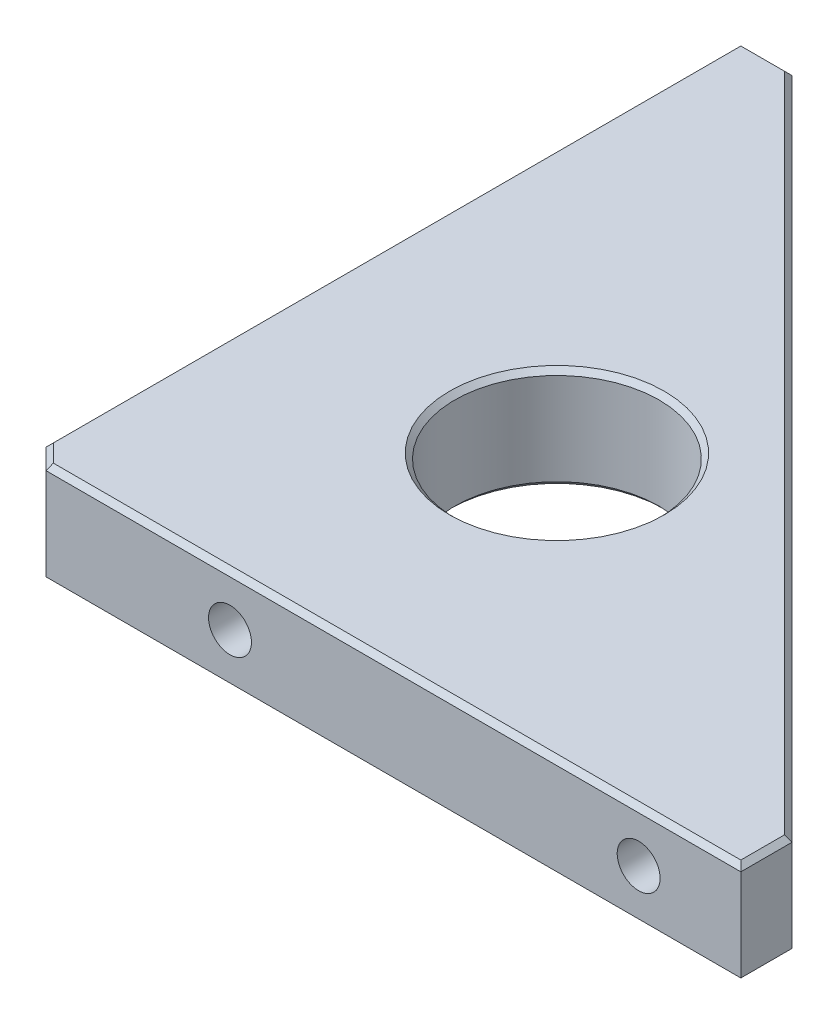
SolidWorks part; units mm, degrees
material "6061 合金"
ref_plane "前视" through (0, 0, 0) normal (0, 0, 1) x (1, 0, 0)
ref_plane "上视" through (0, 0, 0) normal (0, 1, 0) x (1, 0, 0)
ref_plane "右视" through (0, 0, 0) normal (1, 0, 0) x (0, 0, -1)
sketch "草图1" plane through (0, 0, 0) normal (0, 1, 0) x (1, 0, 0)
  line L0 (0, 0) -> (0, 70)
  line L1 (0, 70) -> (5, 70)
  line L2 (5, 70) -> (70, 5)
  line L3 (70, 5) -> (70, 0)
  line L4 (70, 0) -> (0, 0)
  dimension "D1" = 70
  dimension "D2" = 70
  dimension "D3" = 5
  dimension "D4" = 5
extrude "凸台-拉伸1" add sketch "草图1" along normal mid plane 10
chamfer "倒角1" distance 2 angle 45 1 edges at (0, 0, 0)
hole_wizard "M5 螺纹孔1" positions "草图2" profile "草图3" tap size "M5" standard "AS"
sketch "草图2" plane through (0, 0, 0) normal (0, 0, 1) x (1, 0, 0)
  line L0 (0, -5) -> (0, 5) construction
  line L1 (70, 5) -> (70, -5) construction
  point P0 (60, 0)
  point P2 (20, 0)
  dimension "D1" = 20
  dimension "D2" = 10
cosmetic thread "孔螺蚊线1" parameters "D1"=10, "D2"=5
cosmetic thread "孔螺蚊线2" parameters "D1"=10, "D2"=5
sketch "草图3" plane through (60, 0, 0) normal (1, 0, 0) x (0, -1, 0)
  line L0 (0, 0) -> (0, 13.6618)
  line L1 (0, 13.6618) -> (2.1, 12.4)
  line L2 (2.1, 12.4) -> (2.1, 0)
  line L5 (2.1, 0) -> (0, 0)
  line L10 (0, 13.6618) -> (-2.1, 12.4) construction
  line L11 (0, -6.35) -> (0, 107.95) construction
  dimension "螺纹孔钻头直径" = 4.2
  dimension "螺纹孔钻头深度" = 12.4
  dimension "导头角度" = 118
hole_wizard "M5 螺纹孔2" positions "草图4" profile "草图5" tap size "M5" standard "AS"
sketch "草图4" plane through (0, 0, 0) normal (-1, 0, 0) x (0, 0, 1)
  point P0 (-19.0545, 0)
  point P2 (-59.0545, 0)
  dimension "D1" = 19.0545
  dimension "D2" = 40
sketch "草图5" plane through (0, 0, -19.0545) normal (0, 1, 0) x (0, 0, 1)
  line L0 (0, 0) -> (0, 13.6618)
  line L1 (0, 13.6618) -> (2.1, 12.4)
  line L2 (2.1, 12.4) -> (2.1, 0)
  line L5 (2.1, 0) -> (0, 0)
  line L10 (0, 13.6618) -> (-2.1, 12.4) construction
  line L11 (0, -6.35) -> (0, 107.95) construction
  dimension "螺纹孔钻头直径" = 4.2
  dimension "螺纹孔钻头深度" = 12.4
  dimension "导头角度" = 118
cosmetic thread "孔螺蚊线6" parameters "D1"=10, "D2"=5
cosmetic thread "孔螺蚊线7" parameters "D1"=10, "D2"=5
sketch "草图6" plane through (0, -5, 0) normal (0, -1, 0) x (1, 0, 0)
  line L2 (0, -70) -> (0, -2) construction
  line L3 (2, 0) -> (70, 0) construction
  circle A0 centre (26, -26) radius 10
  dimension "D1" = 26
  dimension "D2" = 26
  dimension "D3" = 20
extrude "切除-拉伸1" cut sketch "草图6" against normal through all
chamfer "倒角2" distance 0.5 angle 45 14 edges at (70, -5, -2.5) (37.5, -5, -37.5) (2.5, -5, -70) (0, -5, -36) (1, -5, -1) (36, -5, 0) (2.5, 5, -70) (37.5, 5, -37.5) (70, 5, -2.5) (36, 5, 0) (1, 5, -1) (0, 5, -36) (26, -5, -36) (26, 5, -36)
